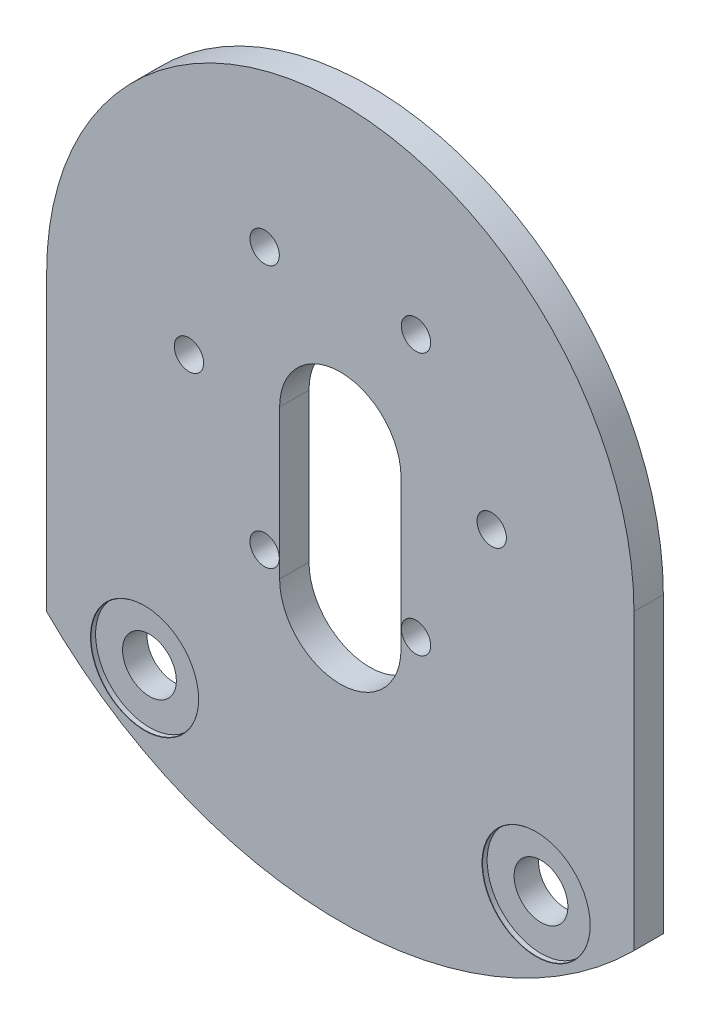
from build123d import *

# Parameters (mm, degrees)
BOSS_EXTRUDE1_DEPTH                          = 3
SKETCH11_R                                   = 1.5
CUT_EXTRUDE1_DEPTH                           = 3
CBORE_FOR_M5_HEXAGON_HEAD_BOLTS_FULL_2_COUNT = 2
CBORE_FOR_M5_HEXAGON_HEAD_BOLTS_FULL_2_PITCH = 40


with BuildPart() as part:
    # Sketch4 → Boss-Extrude1 (new body)
    with BuildSketch(Plane.XY):
        with BuildLine():
            Line((30, 0), (30, -30))
            ThreePointArc((30, -30), (0, -42.426406871), (-30, -30))
            Line((-30, -30), (-30, 0))
            ThreePointArc((-30, 0), (0, 30), (30, 0))
        make_face()
        with BuildLine():
            Line((6.2, 0), (6.2, -15.218791378))
            ThreePointArc((6.2, -15.218791378), (0, -21.418791378), (-6.2, -15.218791378))
            Line((-6.2, -15.218791378), (-6.2, 0))
            ThreePointArc((-6.2, 0), (0, 6.2), (6.2, 0))
        make_face(mode=Mode.SUBTRACT)
    extrude(amount=BOSS_EXTRUDE1_DEPTH)

    # Sketch11 → Cut-Extrude1 (cut)
    with BuildSketch(Plane.XY.offset(3)):
        with Locations((-15.463782922, 0)):
            Circle(SKETCH11_R)
        with Locations((-7.731891461, 13.392028849)):
            Circle(SKETCH11_R)
        with Locations((7.731891461, 13.392028849)):
            Circle(SKETCH11_R)
        with Locations((15.463782922, 0)):
            Circle(SKETCH11_R)
        with Locations((7.731891461, -13.392028849)):
            Circle(SKETCH11_R)
        with Locations((-7.731891461, -13.392028849)):
            Circle(SKETCH11_R)
    extrude(amount=-CUT_EXTRUDE1_DEPTH, mode=Mode.SUBTRACT)

    # Sketch14 → CBORE for M5 Hexagon head bolts-Full thread-grade C1 (revolve, cut)
    with BuildSketch(Plane(origin=(20, -30, 3), x_dir=(0, -1, 0), z_dir=(1, 0, 0))):
        Polygon((0, 0), (0, 3), (2.75, 3), (2.75, 0.5), (5.5, 0.5), (5.5, 0.025), (5.525, 0), align=None)
    cbore_for_m5_hexagon_head_bolts_full_thr = revolve(axis=Axis((20, -30, 9.35), (0, 0, -1)), mode=Mode.SUBTRACT)

    # CBORE for M5 Hexagon head bolts-Full 2: CBORE for M5 Hexagon head bolts-Full thread-grade C1 ×2
    with Locations(*[(-i * CBORE_FOR_M5_HEXAGON_HEAD_BOLTS_FULL_2_PITCH, 0, 0) for i in range(1, CBORE_FOR_M5_HEXAGON_HEAD_BOLTS_FULL_2_COUNT)]):
        add(cbore_for_m5_hexagon_head_bolts_full_thr, mode=Mode.SUBTRACT)


solid = part.part
